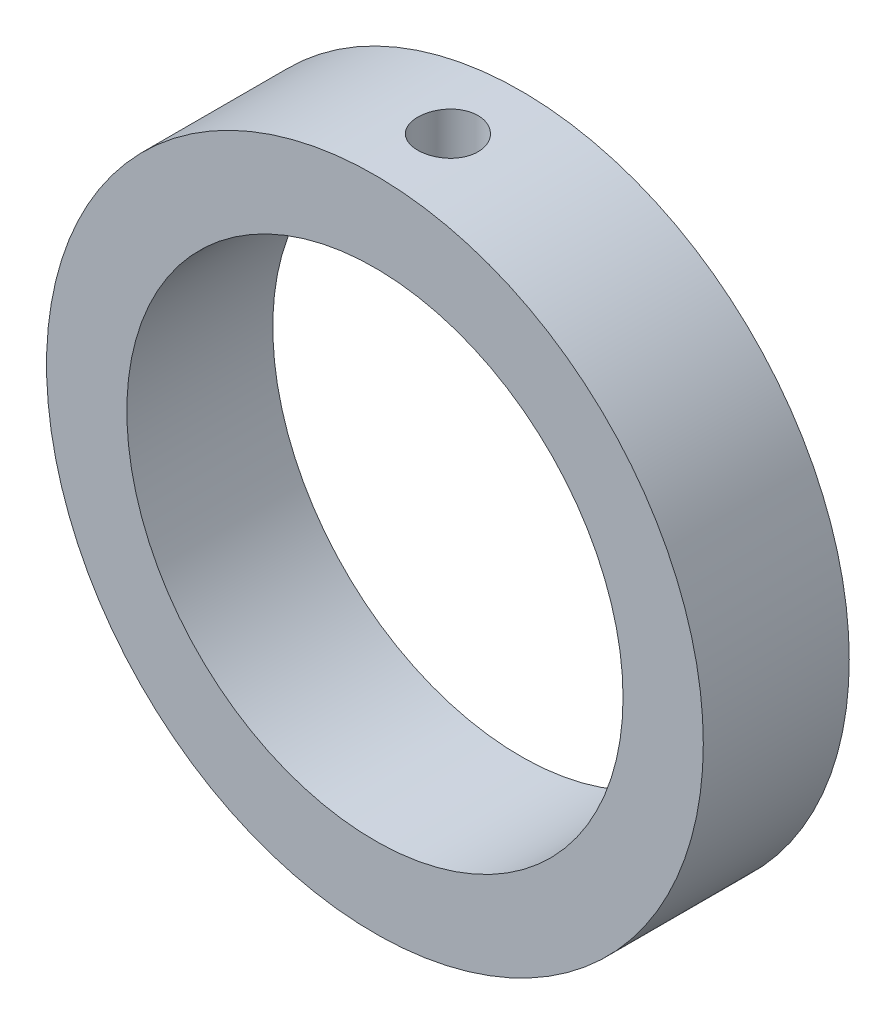
from build123d import *

# Parameters (mm, degrees)
SKETCH_1_R      = 18
SKETCH_1_R_2    = 13.6
EXTRUDE_1_DEPTH = 4
SKETCH_8_W      = 1.65
SKETCH_8_H      = 18


with BuildPart() as part:
    # 草图1 → 凸台-拉伸1 (new, symmetric)
    with BuildSketch(Plane.XY):
        Circle(SKETCH_1_R)
        Circle(SKETCH_1_R_2, mode=Mode.SUBTRACT)
    extrude(amount=EXTRUDE_1_DEPTH, both=True)

    # 草图8 → M4 螺纹孔2 (revolve, cut)
    with BuildSketch(Plane(origin=(0, 0, 0), x_dir=(0, 0, -1), z_dir=(1, 0, 0))):
        with Locations((0.825, 9)):
            Rectangle(SKETCH_8_W, SKETCH_8_H)
    revolve(axis=Axis((0, -6.35, 0), (0, 1, 0)), mode=Mode.SUBTRACT)


solid = part.part
